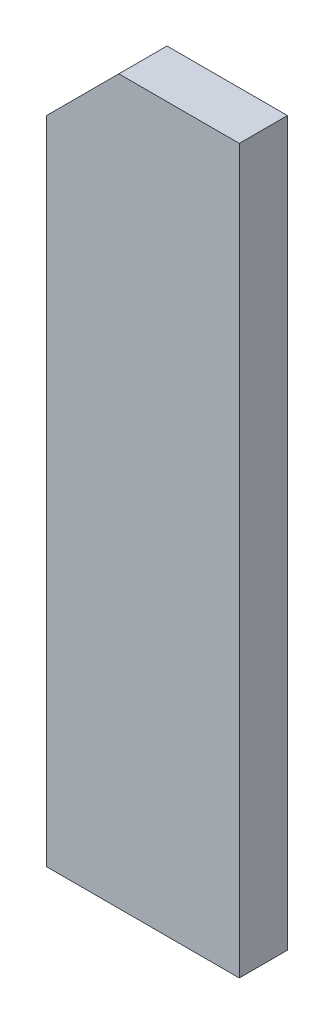
SolidWorks part; units mm, degrees
ref_plane "Front Plane" through (0, 0, 0) normal (0, 0, 1) x (1, 0, 0)
ref_plane "Top Plane" through (0, 0, 0) normal (0, 1, 0) x (1, 0, 0)
ref_plane "Right Plane" through (0, 0, 0) normal (1, 0, 0) x (0, 0, -1)
sketch "Sketch1" plane through (0, 0, 0) normal (0, 0, 1) x (1, 0, 0)
  line L0 (-50, 300) -> (-80, 270)
  line L1 (0, 0) -> (-80, 0)
  line L2 (0, 0) -> (0, 300)
  line L3 (0, 300) -> (-50, 300)
  line L4 (-80, 0) -> (-80, 270)
  dimension "D1" = 80
  dimension "D2" = 50
  dimension "D3" = 270
  dimension "D4" = 300
extrude "Boss-Extrude1" add sketch "Sketch1" along normal blind 20
